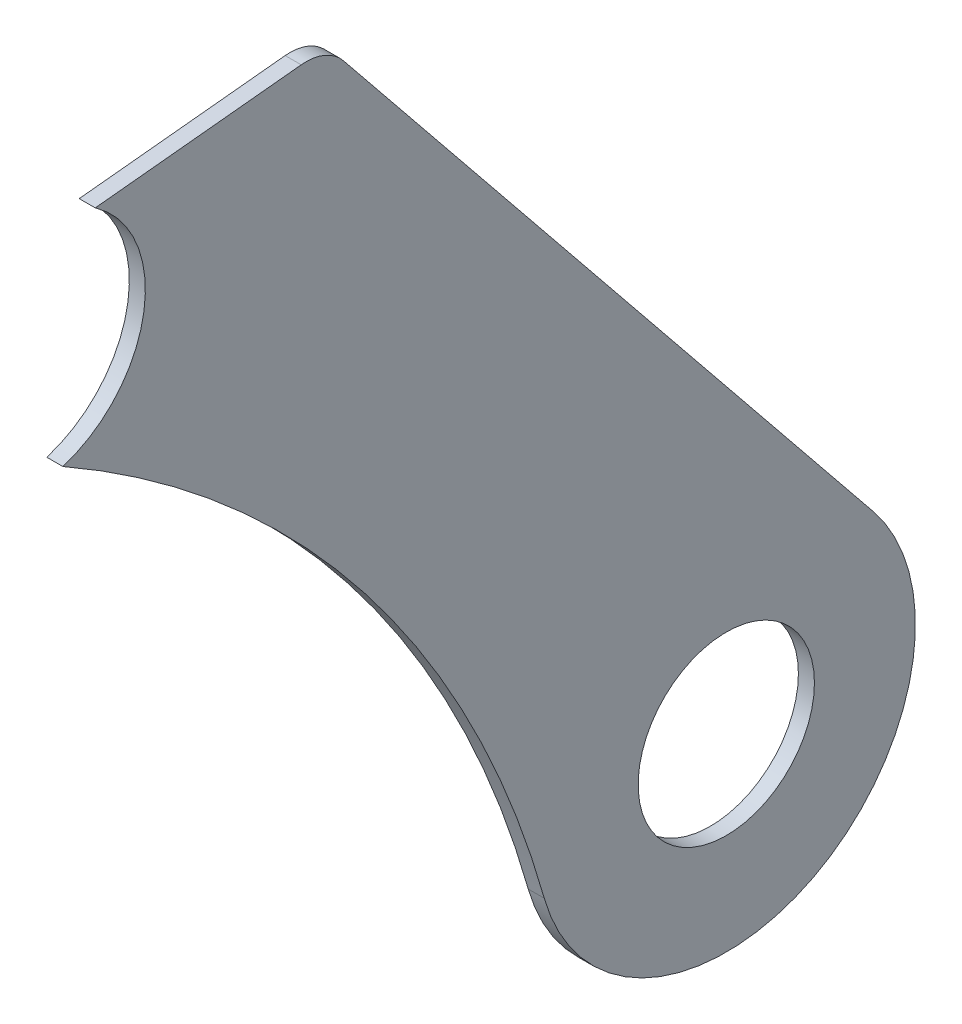
from build123d import *

# Parameters (mm, degrees)
SKETCH1_R           = 55
BOSS_EXTRUDE1_DEPTH = 10


with BuildPart() as part:
    # Sketch1 → Boss-Extrude1 (new body)
    with BuildSketch(Plane(origin=(0, 0, 0), x_dir=(0, 0, -1), z_dir=(1, 0, 0))):
        with BuildLine():
            Line((337.625172258, 687.7), (466.146951534, 700.758734438))
            ThreePointArc((466.146951534, 700.758734438), (480.718476107, 698.604521018), (492.508223096, 689.774355121))
            Line((492.508223096, 689.774355121), (823.174539509, 280.80254433))
            ThreePointArc((823.174539509, 280.80254433), (785.648592785, 101.78743459), (617.824738614, 174.518171996))
            ThreePointArc((617.824738614, 174.518171996), (505.411922854, 395.882290886), (317.415259146, 558.042608823))
            ThreePointArc((317.415259146, 558.042608823), (368.029035851, 616.55712727), (337.625172258, 687.7))
        make_face()
        with Locations((731.4, 206.6)):
            Circle(SKETCH1_R, mode=Mode.SUBTRACT)
    extrude(amount=BOSS_EXTRUDE1_DEPTH)


solid = part.part
